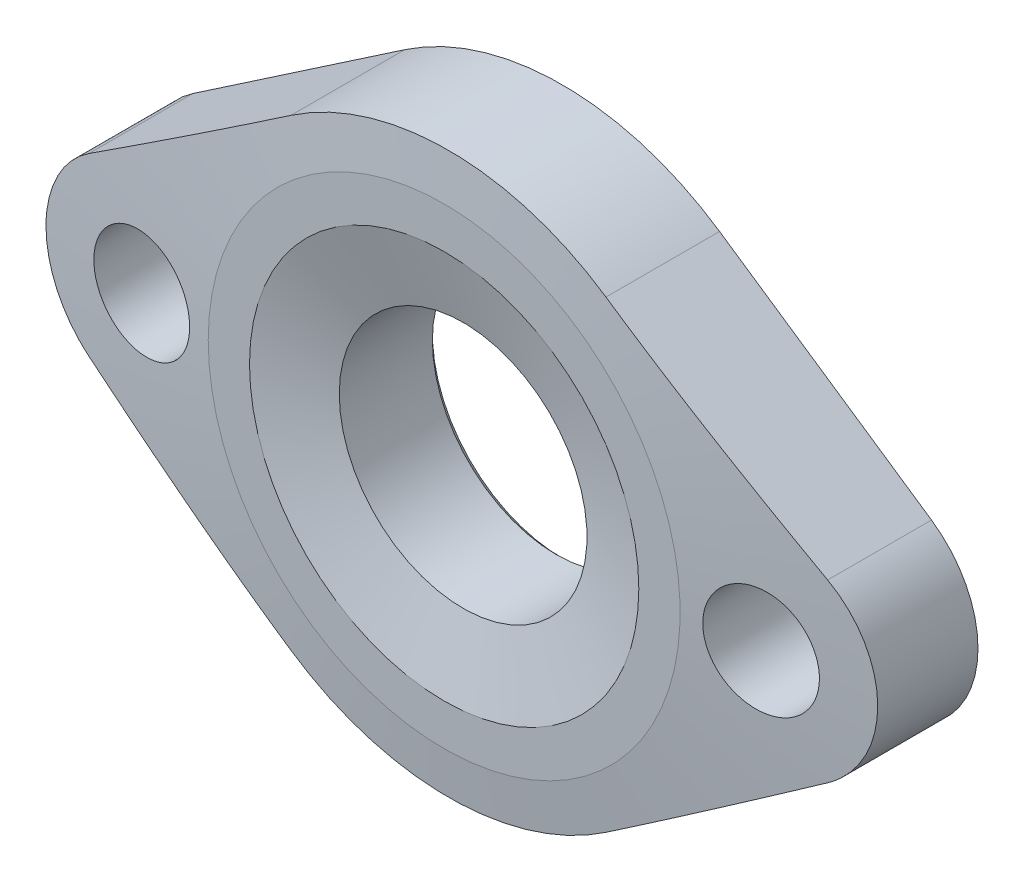
SolidWorks part; units mm, degrees
ref_plane "Front Plane" through (0, 0, 0) normal (0, 0, 1) x (1, 0, 0)
ref_plane "Top Plane" through (0, 0, 0) normal (0, 1, 0) x (1, 0, 0)
ref_plane "Right Plane" through (0, 0, 0) normal (1, 0, 0) x (0, 0, -1)
sketch "Sketch1" plane through (0, 0, 0) normal (0, 0, 1) x (1, 0, 0)
  line L0 (0, 0) -> (52.5, 0) construction
  line L1 (26.6905, 39.2921) -> (62.6143, 14.8896)
  line L2 (26.6905, -39.2921) -> (62.6143, -14.8896)
  line L3 (0, 0) -> (0, -91.5706) construction
  line L4 (0, 0) -> (-52.5, 0) construction
  line L5 (-26.6905, -39.2921) -> (-62.6143, -14.8896)
  line L6 (-26.6905, 39.2921) -> (-62.6143, 14.8896)
  arc A0 (26.6905, 39.2921) -> (-26.6905, 39.2921) centre (0, 0) ccw
  arc A1 (62.6143, -14.8896) -> (62.6143, 14.8896) centre (52.5, 0) ccw
  arc A2 (-62.6143, -14.8896) -> (-62.6143, 14.8896) centre (-52.5, 0) cw
  arc A3 (-26.6905, 39.2921) -> (26.6905, 39.2921) centre (0, 0) cw
  circle A4 centre (52.5, 0) radius 9
  circle A5 centre (-52.5, 0) radius 9
  arc A6 (46.9667, -7.098) -> (26.6905, -39.2921) centre (0, 0) cw construction
  arc A7 (26.6905, -39.2921) -> (-26.6905, -39.2921) centre (0, 0) cw
  arc A8 (26.6905, 39.2921) -> (46.9667, 7.098) centre (0, 0) cw construction
  arc A9 (47.5, 0) -> (46.9667, -7.098) centre (0, 0) cw construction
  arc A10 (46.9667, 7.098) -> (47.5, 0) centre (0, 0) cw construction
  arc A11 (-26.6905, 39.2921) -> (-46.9667, 7.098) centre (0, 0) ccw construction
  arc A12 (-46.9667, 7.098) -> (26.6905, -39.2921) centre (0, 0) ccw
  point P3 (26.25, 0)
  point P14 (-26.25, 0)
  dimension "D1" = 18
  dimension "D2" = 47.5
  dimension "D3" = 18
  dimension "D4" = 105
extrude "Boss-Extrude1" add sketch "Sketch1" along normal blind 20
sketch "Sketch5" plane through (0, 0, 0) normal (0, 1, 0) x (1, 0, 0)
  line L0 (26.6905, -20) -> (62.6143, -20) construction
  line L1 (0, 0) -> (21, 0)
  line L2 (0, 0) -> (0, -16.7846)
  line L3 (0, -16.7846) -> (21, -16.7846)
  line L4 (21, 0) -> (21, -16.7846)
  line L5 (0, -16.7846) -> (21, -16.7846)
  line L6 (0, -16.7846) -> (0, -20)
  line L7 (0, -20) -> (33, -20)
  line L8 (21, -16.7846) -> (33, -20)
  line L9 (40, -20) -> (70.5, -17)
  line L10 (70.5, -20) -> (70.5, 0) construction
  line L11 (-52.25, 0) -> (52.25, 0) construction
  line L12 (40, -20) -> (70.5, -20)
  line L13 (70.5, -20) -> (70.5, -17)
  dimension "D1" = 33
  dimension "D2" = 21
  dimension "D3" = 15
  dimension "D4" = 17
  dimension "D5" = 40
revolve "Cut-Revolve1" cut sketch "Sketch5" angle 360 about L2
chamfer "Chamfer1" distance 1 angle 45 1 edges at (-21, 0, 0)
